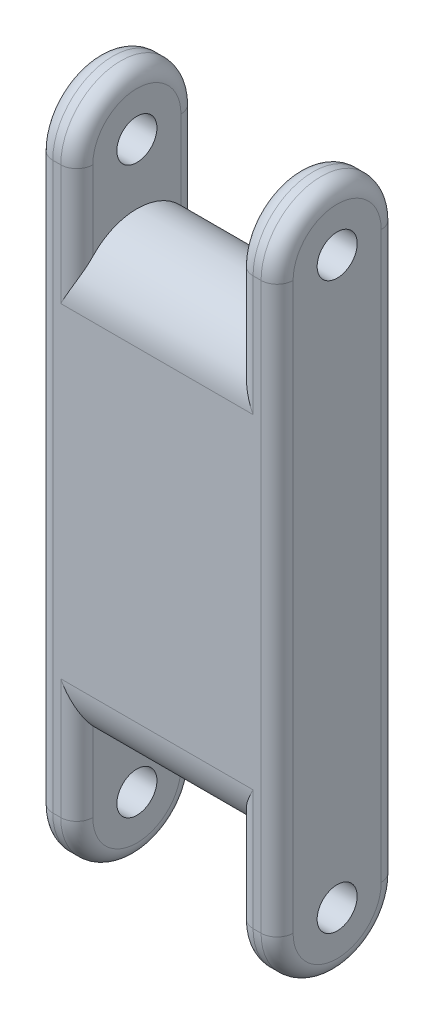
SolidWorks part; units mm, degrees
material "ABS"
ref_plane "Front" through (0, 0, 0) normal (0, 0, 1) x (1, 0, 0)
ref_plane "Top" through (0, 0, 0) normal (0, 1, 0) x (1, 0, 0)
ref_plane "Right" through (0, 0, 0) normal (1, 0, 0) x (0, 0, -1)
sketch "Sketch1" plane through (0, 0, 0) normal (1, 0, 0) x (0, 0, -1)
  line L0 (-4.7625, 0) -> (-4.7625, 44.8056)
  line L1 (4.7625, 44.8056) -> (4.7625, 0)
  arc A0 (-4.7625, 44.8056) -> (4.7625, 44.8056) centre (0, 44.8056) cw
  arc A1 (4.7625, 0) -> (-4.7625, 0) centre (0, 0) cw
  dimension "D1" = 9.525
  dimension "D2" = 44.8056
extrude "Boss-Extrude1" add sketch "Sketch1" along normal blind 19.05
sketch "Sketch2" plane through (19.05, 0, 0) normal (1, 0, 0) x (0, 0, -1)
  circle A0 centre (0, 0) radius 1.5875
  circle A1 centre (0, 44.8056) radius 1.5875
  dimension "D1" = 3.175
extrude "Cut-Extrude1" cut sketch "Sketch2" against normal blind 19.05
sketch3d "3DSketch1"
  line L0 (9.525, 44.8056, -4.7625) -> (9.525, 35.2806, -4.7625)
  line L1 (19.05, 44.8056, -4.7625) -> (0, 44.8056, -4.7625) construction
  line L2 (19.05, 44.8056, 4.7625) -> (0, 44.8056, 4.7625) construction
  line L3 (9.525, 44.8056, 4.7625) -> (9.525, 35.2806, 4.7625)
  line L5 (9.525, 0, 4.7625) -> (9.525, 9.525, 4.7625)
  line L7 (19.05, 0, 4.7625) -> (0, 0, 4.7625) construction
  line L8 (19.05, 0, -4.7625) -> (0, 0, -4.7625) construction
  line L9 (9.525, 0, -4.7625) -> (9.525, 9.525, -4.7625)
  arc A0 (9.525, 44.8056, -4.7625) -> (9.525, 44.8056, 4.7625) centre (9.525, 44.8056, 0) ccw
  arc A1 (9.525, 35.2806, -4.7625) -> (9.525, 35.2806, 4.7625) centre (9.525, 35.2806, 0) cw
  arc A2 (9.525, 0, 4.7625) -> (9.525, 0, -4.7625) centre (9.525, 0, 0) ccw
  arc A3 (9.525, 9.525, -4.7625) -> (9.525, 9.525, 4.7625) centre (9.525, 9.525, 0) cw
  point P6 (14.2875, 44.8056, 0)
  point P12 (14.2875, 35.2806, 0)
  point P18 (14.2875, 0, 0)
  point P24 (4.7625, 9.525, 0)
  dimension "D1" = 9.525
  dimension "D2" = 9.525
extrude "Cut-Extrude2" cut sketch "3DSketch1" along direction (-1, 0, 0) on the side against the normal mid plane 12.7
fillet "Fillet1" radius 1.27 20 edges at (0, 49.5681, 0) (0, 22.4028, -4.7625) (0, -4.7625, 0) (19.05, 49.5681, 0) (19.05, 22.4028, -4.7625) (19.05, -4.7625, 0) (0, 22.4028, 4.7625) (19.05, 22.4028, 4.7625)
sketch "Sketch3" plane through (0, 0, 0) normal (-1, 0, 0) x (0, 0, 1)
  line L0 (-3.4925, 44.8056) -> (-3.4925, 0) construction
  circle A0 centre (-2.0685, 42.4909) radius 1.3523
  circle A2 centre (0, 44.8056) radius 1.5875 construction
  dimension "D1" = 2.7047
  dimension "D2" = 1.424
  dimension "D3" = 2.3147
extrude "Boss-Extrude2" add sketch "Sketch3" along normal blind 2.54
fillet "Fillet2" radius 0.762 1 edges at (-2.54, 42.4909, -0.7161)
ref_plane "Plane1" through (0, 10.4032, 18.0189) normal (0, 0.5, 0.866) x (-1, 0, 0)
sketch "Sketch4" plane through (0, 10.4032, 18.0189) normal (0, 0.5, 0.866) x (-1, 0, 0)
  line L0 (0, -40.549) -> (0, -1.7462) construction
  line L2 (-1.905, -28.1726) -> (-17.145, -28.1726) construction
  circle A0 centre (0.8782, -37.9336) radius 0.6365
  dimension "D1" = 1.2731
  dimension "D2" = 0.8782
  dimension "D3" = 9.761
extrude "Cut-Extrude3" cut sketch "Sketch4" against normal through all
scale "Scale ratio 1" scale about origin uniform scaling yes scale factor 1.3
